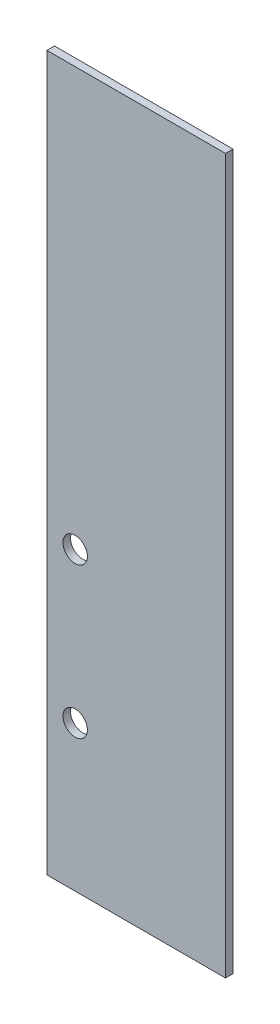
from build123d import *

# Parameters (mm, degrees)
SKETCH_1_W      = 95
SKETCH_1_H      = 380
SKETCH_1_R      = 6.5
EXTRUDE_2_DEPTH = 4


with BuildPart() as part:
    # 草图1 → 凸台-拉伸2 (new body)
    with BuildSketch(Plane.XY):
        with Locations((47.5, -190)):
            Rectangle(SKETCH_1_W, SKETCH_1_H)
        with Locations((15, -302.5)):
            Circle(SKETCH_1_R, mode=Mode.SUBTRACT)
        with Locations((15, -222.5)):
            Circle(SKETCH_1_R, mode=Mode.SUBTRACT)
    extrude(amount=EXTRUDE_2_DEPTH)


solid = part.part
